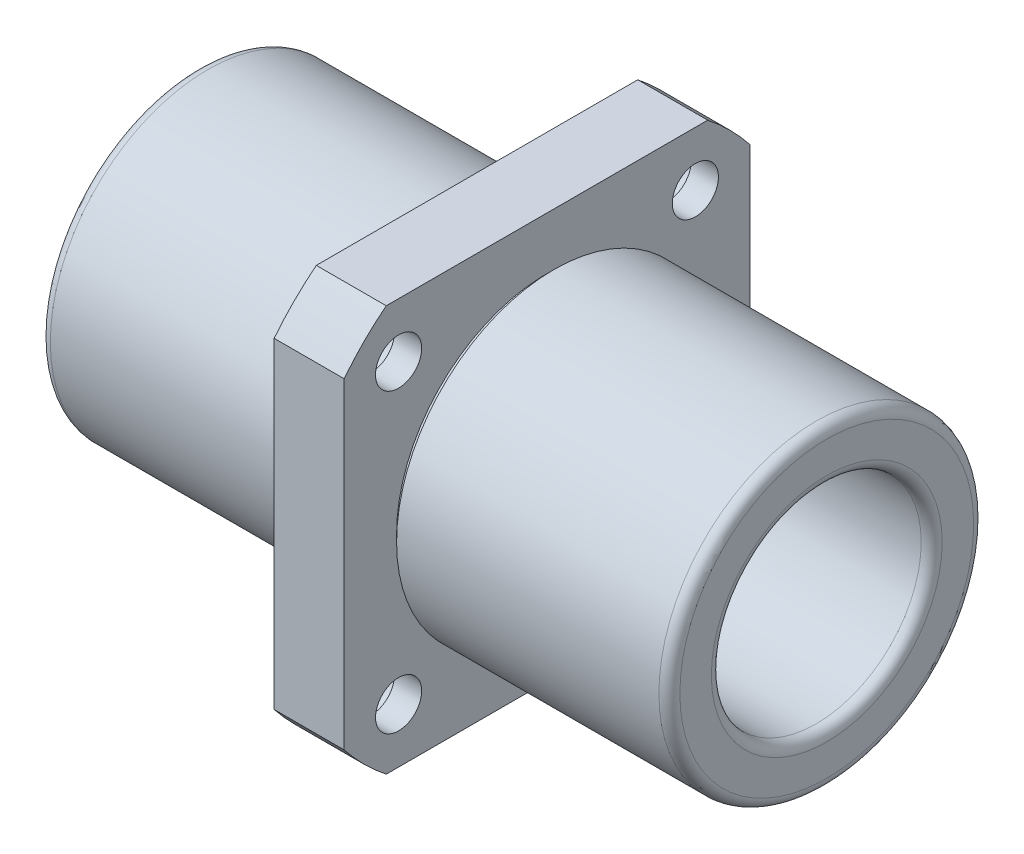
from build123d import *

# Parameters (mm, degrees)
SKETCH2_OUTSIDE_W   = 103.606
SKETCH2_OUTSIDE_H   = 103.606
SKETCH2_OUTSIDE_W_2 = 58
SKETCH2_OUTSIDE_H_2 = 58
CUT_EXTRUDE1_DEPTH  = 10
SKETCH3_R           = 5.5
CUT_EXTRUDE2_DEPTH  = 6.1
CUT_EXTRUDE3_REACH  = 63.703
SKETCH4_R           = 3.3
CIRPATTERN1_COUNT   = 4
FILLET1_R           = 1.5


with BuildPart() as part:
    # Sketch1 → Revolve1 (revolve)
    with BuildSketch(Plane.XY, mode=Mode.PRIVATE) as revolve1_sk:
        Polygon((0, 37), (0, 21.5), (-1, 21.5), (-1, 22.5), (-40, 22.5), (-40, 15), (0, 15), (50, 15), (50, 22.5), (11, 22.5), (11, 21.5), (10, 21.5), (10, 37), align=None)
    revolve(revolve1_sk.sketch.rotate(Axis((64, 0, 0), (-1, 0, 0)), 270), axis=Axis((64, 0, 0), (-1, 0, 0)))

    # Sketch2 outside → Cut-Extrude1 (cut)
    with BuildSketch(Plane(origin=(0, 0, 0), x_dir=(0, 0, -1), z_dir=(1, 0, 0))):
        Rectangle(SKETCH2_OUTSIDE_W, SKETCH2_OUTSIDE_H)
        Rectangle(SKETCH2_OUTSIDE_W_2, SKETCH2_OUTSIDE_H_2, mode=Mode.SUBTRACT)
    extrude(amount=CUT_EXTRUDE1_DEPTH, mode=Mode.SUBTRACT)

    # Sketch3 → Cut-Extrude2 (cut)
    with BuildSketch(Plane.ZY):
        with Locations((-21.213203436, 21.213203436)):
            Circle(SKETCH3_R)
    cut_extrude2 = extrude(amount=-CUT_EXTRUDE2_DEPTH, mode=Mode.SUBTRACT)

    # Sketch4 → Cut-Extrude3 (cut, up to next)
    with BuildSketch(Plane.ZY.offset(-6.1), mode=Mode.PRIVATE) as cut_extrude3_sk1:
        with Locations((-21.213203436, 21.213203436)):
            Circle(SKETCH4_R)
    cut_extrude3_tool1 = extrude(cut_extrude3_sk1.sketch, amount=-CUT_EXTRUDE3_REACH, mode=Mode.PRIVATE) & part.part
    cut_extrude3 = cut_extrude3_tool1.solids().sort_by_distance((6.1, 21.213203, -21.213203))[0]
    add(cut_extrude3, mode=Mode.SUBTRACT)

    # CirPattern1: Cut-Extrude2, Cut-Extrude3 ×4 about axis
    cirpattern1_axis = Axis((0, 0, 0), (1, 0, 0))
    add([cut_extrude2.rotate(cirpattern1_axis, i * 360 / CIRPATTERN1_COUNT) for i in range(1, CIRPATTERN1_COUNT)], mode=Mode.SUBTRACT)
    add([cut_extrude3.rotate(cirpattern1_axis, i * 360 / CIRPATTERN1_COUNT) for i in range(1, CIRPATTERN1_COUNT)], mode=Mode.SUBTRACT)

    # Fillet1
    fillet1_edges = [part.edges().sort_by_distance(p)[0] for p in [
        (50, 0, -22.5),
        (50, 0, -15),
        (-40, 0, -15),
        (-40, 0, -22.5),
    ]]
    fillet(fillet1_edges, radius=FILLET1_R)


solid = part.part
